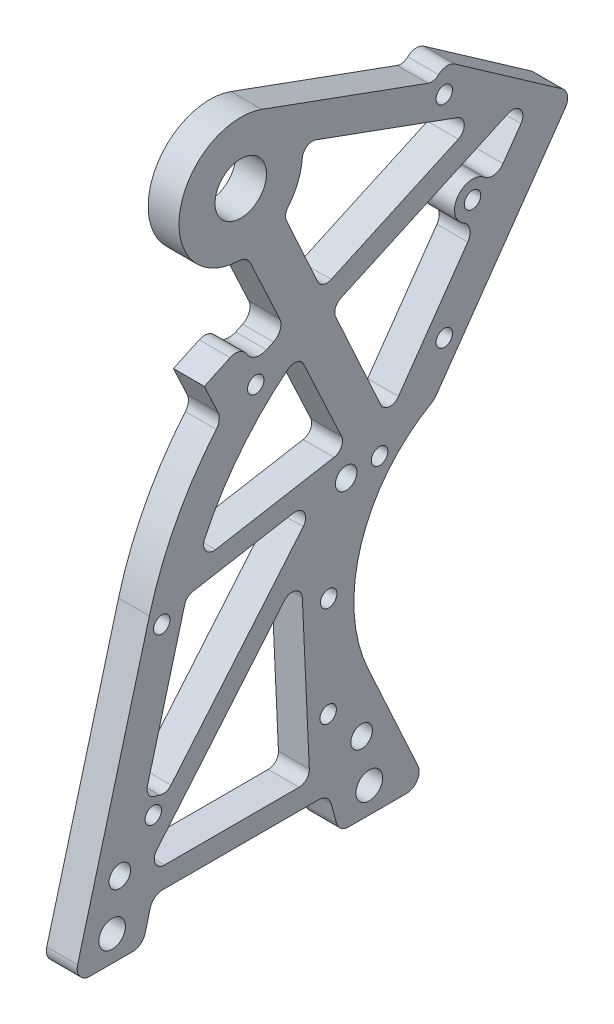
SolidWorks part; units mm, degrees
material "Thornel Mat VMA"
ref_plane "前视基准面" through (0, 0, 0) normal (0, 0, 1) x (1, 0, 0)
ref_plane "上视基准面" through (0, 0, 0) normal (0, 1, 0) x (1, 0, 0)
ref_plane "右视基准面" through (0, 0, 0) normal (1, 0, 0) x (0, 0, -1)
sketch "草图1" plane through (0, 0, 0) normal (1, 0, 0) x (0, 0, -1)
  line L0 (-17.0832, 0) -> (17.0832, 0)
  line L1 (-32.5618, -7.5) -> (-19.0928, -7.5)
  line L2 (-17.0832, 0) -> (-19.0928, -7.5)
  line L3 (17.0832, 0) -> (19.0928, -7.5)
  line L4 (0, 0) -> (0, -7.5) construction
  line L5 (19.0928, -7.5) -> (36.0897, -7.5)
  line L6 (1.1561, 98.5558) -> (8.6307, 82.5266)
  line L7 (8.6307, 82.5266) -> (5.0055, 80.8361)
  line L8 (-5, 110.5) -> (5, 110.5) construction
  line L9 (36.0897, -7.5) -> (24.7253, 17.3094)
  line L10 (4.1042, 121.7763) -> (36.4214, 110.0138)
  line L12 (41.617, 110.6581) -> (64.5533, 94.5979)
  line L13 (64.5533, 94.5979) -> (37.6186, 56.1313)
  line L14 (-32.5618, -7.5) -> (-17.7603, 47.4158)
  line L16 (-2.0717, 83.0529) -> (-7.077, 80.7189)
  line L17 (-7.077, 80.7189) -> (-3.7224, 73.5248)
  circle A0 centre (0, 110.5) radius 5
  circle A1 centre (52, 29.803) radius 28.5 construction
  circle A2 centre (-25, -2.5) radius 2.6
  circle A3 centre (25, -2.5) radius 2.6
  arc A4 (4.1042, 121.7763) -> (1.1561, 98.5558) centre (0, 110.5) ccw
  arc A5 (37.6186, 56.1313) -> (24.7253, 17.3094) centre (52, 29.803) ccw
  arc A8 (-3.7224, 73.5248) -> (-17.7603, 47.4158) centre (45, 30.5) ccw
  arc A10 (5.0055, 80.8361) -> (1.1452, 82.0453) centre (3.7376, 83.5551) cw
  arc A11 (1.1452, 82.0453) -> (-2.0717, 83.0529) centre (-1.0151, 80.7871) ccw
  arc A12 (36.4214, 110.0138) -> (38.4733, 110.4341) centre (37.1055, 111.8932) ccw
  arc A13 (41.617, 110.6581) -> (38.4733, 110.4341) centre (40.1831, 108.6102) ccw
  point P3 (0, 0)
  dimension "D2" = 10
  dimension "D3" = 57
  dimension "D8" = 5.2
  dimension "D10" = 24
  dimension "D13" = 30
  dimension "D16" = 35
  dimension "D19" = 65
  dimension "D25" = 2.5
  dimension "D26" = 3
  dimension "D28" = 2
  dimension "D29" = 2.5
  dimension "D1" = 110.5
  dimension "D4" = 7.5
  dimension "D5" = 50
  dimension "D6" = 50
  dimension "D7" = 2.5
  dimension "D9" = 7
  dimension "D11" = 29
  dimension "D12" = 65
  dimension "D14" = 52
  dimension "D15" = 96
  dimension "D17" = 24
  dimension "D18" = 62
  dimension "D20" = 7
  dimension "D21" = 6
  dimension "D22" = 5
  dimension "D23" = 15
  dimension "D24" = 4
  dimension "D27" = 4
  dimension "D30" = 80
  dimension "D31" = 28
  dimension "D32" = 15
  dimension "D33" = 105
  dimension "D34" = 8
extrude "凸台-拉伸1" add sketch "草图1" along normal blind 6
sketch "草图2" plane through (6, 0, 0) normal (1, 0, 0) x (0, 0, -1)
  line L0 (-17, 13.5) -> (17, 13.5) construction
  line L1 (-17.0832, 0) -> (17.0832, 0) construction
  line L2 (45, 30.5) -> (17.1065, 32.9404) construction
  line L3 (45, 30.5) -> (27.0019, 51.9492) construction
  line L4 (2.9189, 76.0322) -> (27.0019, 51.9492) construction
  line L5 (17.1065, 32.9404) -> (-15.3402, 44.75) construction
  line L6 (4.0735, 86.0519) -> (45.0735, 86.0519) construction
  line L7 (4.0735, 86.0519) -> (39.5805, 106.5519) construction
  line L8 (4.0735, 86.0519) -> (39.5805, 65.5519) construction
  line L9 (45, 30.5) -> (22.0081, 30.5) construction
  line L10 (0, 30.5) -> (0, 0) construction
  line L11 (0, 110.5) -> (6.1652, 109.9606) construction
  line L12 (0, 110.5) -> (5, 110.5) construction
  line L13 (-23.5, 6.5) -> (23.5, 6.5) construction
  circle A0 centre (-17, 13.5) radius 1.6
  circle A1 centre (17, 13.5) radius 1.6
  arc A2 (39.5805, 106.5519) -> (39.5805, 65.5519) centre (4.0735, 86.0519) cw construction
  circle A3 centre (39.5805, 106.5519) radius 1.6
  circle A4 centre (45.0735, 86.0519) radius 1.6
  circle A5 centre (39.5805, 65.5519) radius 1.6
  arc A6 (27.0019, 51.9492) -> (17.1065, 32.9404) centre (45, 30.5) ccw construction
  circle A7 centre (27.0019, 51.9492) radius 1.6
  circle A8 centre (17.1065, 32.9404) radius 1.6
  circle A9 centre (2.9189, 76.0322) radius 1.6
  circle A10 centre (-15.3402, 44.75) radius 1.6
  arc A11 (-15.3402, 44.75) -> (2.9189, 76.0322) centre (45, 30.5) cw construction
  arc A12 (37.6186, 56.1313) -> (24.7253, 17.3094) centre (52, 29.803) ccw construction
  arc A13 (18.3088, 66.7295) -> (0, 30.5) centre (45, 30.5) ccw construction
  arc A14 (18.3088, 66.7295) -> (6.1652, 109.9606) centre (4.0735, 86.0519) ccw construction
  circle A15 centre (0, 110.5) radius 5 construction
  circle A16 centre (-23.5, 6.5) radius 2.1
  circle A17 centre (23.5, 6.5) radius 2.1
  circle A18 centre (20.5, 51.5) radius 2.1
  point P4 (0, 13.5)
  point P32 (0, 110.5)
  point P44 (0, 0)
  dimension "D1" = 3.2
  dimension "D4" = 41
  dimension "D5" = 62
  dimension "D6" = 28
  dimension "D12" = 90
  dimension "D13" = 48
  dimension "D16" = 4.2
  dimension "D19" = 45
  dimension "D2" = 34
  dimension "D3" = 13.5
  dimension "D7" = 30
  dimension "D8" = 165
  dimension "D9" = 175
  dimension "D10" = 5
  dimension "D11" = 45
  dimension "D14" = 80
  dimension "D15" = 5
  dimension "D17" = 47
  dimension "D18" = 6.5
  dimension "D20" = 3
extrude "切除-拉伸1" cut sketch "草图2" against normal through all
sketch "草图3" plane through (6, 0, 0) normal (1, 0, 0) x (0, 0, -1)
  line L0 (0, 110.5) -> (27.0019, 51.9492) construction
  line L1 (12.2484, 74.7684) -> (19.6111, 58.9791)
  line L2 (1.1561, 98.5558) -> (8.6307, 82.5266) construction
  line L3 (8.888, 100.651) -> (14.9396, 87.3816)
  line L4 (-4.8845, 52.1371) -> (18.143, 56.1637)
  line L5 (17.5892, 86.3917) -> (42.2978, 97.6602)
  line L6 (42.1519, 101.3593) -> (14.6476, 111.3701)
  line L7 (19.4564, 82.2974) -> (52.0306, 97.1531)
  line L8 (54.4988, 94.1862) -> (48.5556, 85.6984)
  line L9 (18.4666, 79.6479) -> (27.2118, 60.4722)
  line L10 (37.6186, 56.1313) -> (64.5533, 94.5979) construction
  line L11 (46.5966, 82.9008) -> (30.6698, 60.1549)
  line L12 (10.2828, 50.7286) -> (-9.3137, 47.3019)
  line L13 (-10.9003, 45.8523) -> (-18.1489, 18.9589)
  line L14 (-13.5511, 16.8324) -> (12.1593, 47.4729)
  line L15 (-14.8081, 4) -> (11.3387, 4)
  line L16 (13.3366, 6.0919) -> (11.9774, 35.6326)
  line L17 (8.4474, 36.8263) -> (-16.3402, 7.2856)
  line L18 (-17.0832, 0) -> (17.0832, 0) construction
  line L19 (-17.7603, 47.4158) -> (-32.5618, -7.5) construction
  line L20 (36.4214, 110.0138) -> (4.1042, 121.7763) construction
  arc A0 (4.1042, 121.7763) -> (1.1561, 98.5558) centre (0, 110.5) ccw construction
  arc A1 (9.1781, 102.7693) -> (11.9688, 109.6349) centre (0, 110.5) ccw
  arc A2 (9.1903, 75.4879) -> (-7.039, 54.9579) centre (45, 30.5) ccw
  arc A3 (-3.7224, 73.5248) -> (-17.7603, 47.4158) centre (45, 30.5) ccw construction
  arc A4 (48.5556, 85.6984) -> (46.5966, 82.9008) centre (45.0735, 86.0519) ccw
  arc A5 (-7.039, 54.9579) -> (-4.8845, 52.1371) centre (-5.229, 54.1072) ccw
  arc A6 (19.6111, 58.9791) -> (18.143, 56.1637) centre (17.7985, 58.1338) cw
  arc A7 (12.2484, 74.7684) -> (9.1903, 75.4879) centre (10.4358, 73.9231) ccw
  arc A8 (17.5892, 86.3917) -> (14.9396, 87.3816) centre (16.7593, 88.2114) cw
  arc A9 (8.888, 100.651) -> (9.1781, 102.7693) centre (10.7077, 101.4809) cw
  arc A10 (14.6476, 111.3701) -> (11.9688, 109.6349) centre (13.9636, 109.4907) ccw
  arc A11 (42.2978, 97.6602) -> (42.1519, 101.3593) centre (41.4679, 99.4799) ccw
  arc A12 (19.4564, 82.2974) -> (18.4666, 79.6479) centre (20.2863, 80.4777) ccw
  arc A13 (27.2118, 60.4722) -> (30.6698, 60.1549) centre (29.0315, 61.3021) ccw
  arc A14 (52.0306, 97.1531) -> (54.4988, 94.1862) centre (52.8605, 95.3334) cw
  arc A15 (-15.8499, 16.2708) -> (-16.5307, 16.4631) centre (-17, 13.5) ccw
  arc A16 (-9.3137, 47.3019) -> (-10.9003, 45.8523) centre (-8.9692, 45.3318) ccw
  arc A17 (10.2828, 50.7286) -> (12.1593, 47.4729) centre (10.6273, 48.7585) cw
  arc A18 (11.9774, 35.6326) -> (8.4474, 36.8263) centre (9.9795, 35.5407) ccw
  arc A19 (11.3387, 4) -> (13.3366, 6.0919) centre (11.3387, 6) ccw
  arc A20 (-14.8081, 4) -> (-16.3402, 7.2856) centre (-14.8081, 6) cw
  arc A21 (-18.1489, 18.9589) -> (-16.5307, 16.4631) centre (-16.2178, 18.4384) ccw
  arc A22 (-15.8499, 16.2708) -> (-13.5511, 16.8324) centre (-15.0832, 18.118) ccw
  point P11 (20.5, 51.5)
  point P30 (-8.528, 51.5)
  point P45 (17.6367, 81.4675)
  point P64 (-15.3402, 44.75)
  point P65 (17, 13.5)
  point P69 (39.5805, 106.5519)
  point P85 (17.1065, 32.9404)
  dimension "D1" = 57.5
  dimension "D5" = 3.5
  dimension "D6" = 2
  dimension "D7" = 4
  dimension "D11" = 6
  dimension "D13" = 2
  dimension "D2" = 5
  dimension "D3" = 8
  dimension "D4" = 4.5
  dimension "D8" = 4
  dimension "D9" = 4
  dimension "D10" = 4
  dimension "D12" = 4
  dimension "D14" = 5
  dimension "D15" = 50
  dimension "D16" = 4.5
  dimension "D17" = 4
extrude "切除-拉伸2" cut sketch "草图3" against normal through all
fillet "R2.5 圆角1" radius 2.5 13 edges at (3, 85.6984, -48.5556) (3, 82.9008, -46.5966) (3, 94.5979, -64.5533) (3, 56.1313, -37.6186) (3, -7.5, -36.0897) (3, -7.5, -19.0928) (3, 0, -17.0832) (3, 0, 17.0832) (3, -7.5, 19.0928) (3, -7.5, 32.5618) (3, 73.5248, 3.7224) (3, 98.5558, -1.1561) (3, 82.5266, -8.6307)
